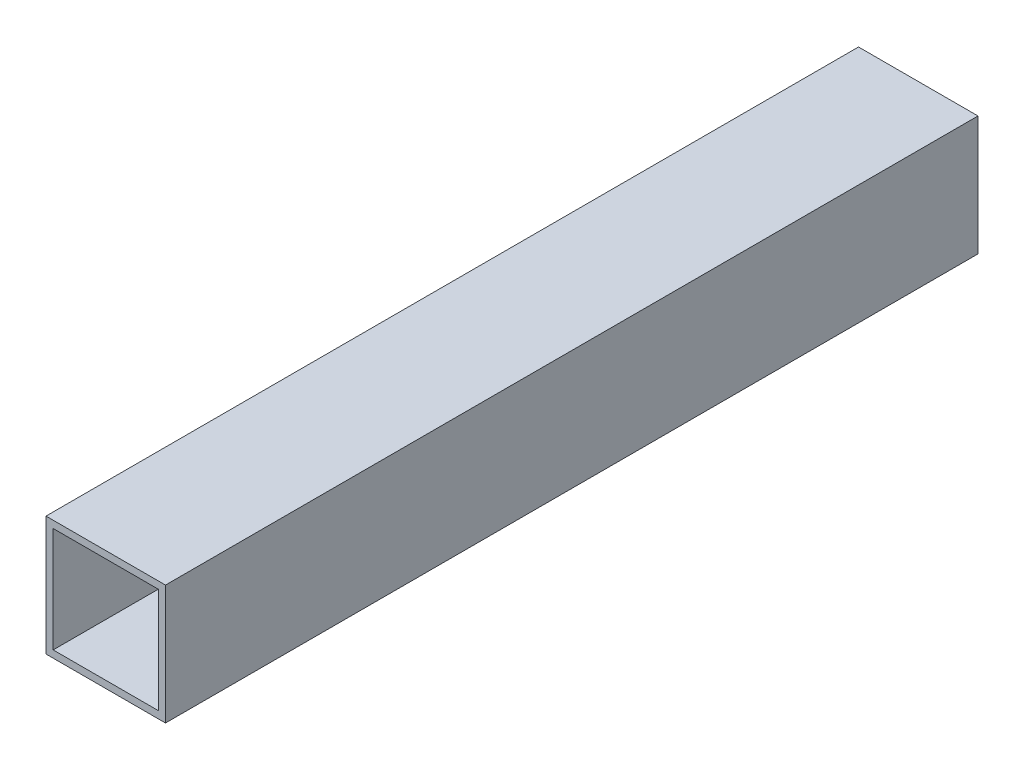
SolidWorks part; units mm, degrees
ref_plane "前视基准面" through (0, 0, 0) normal (0, 0, 1) x (1, 0, 0)
ref_plane "上视基准面" through (0, 0, 0) normal (0, 1, 0) x (1, 0, 0)
ref_plane "右视基准面" through (0, 0, 0) normal (1, 0, 0) x (0, 0, -1)
sketch "草图1" plane through (0, 0, 0) normal (0, 0, 1) x (1, 0, 0)
  line L0 (0, 0) -> (0, 50)
  line L1 (0, 50) -> (50, 50)
  line L2 (50, 50) -> (50, 0)
  line L3 (50, 0) -> (0, 0)
  line L4 (3, 3) -> (3, 47)
  line L5 (3, 47) -> (47, 47)
  line L6 (47, 47) -> (47, 3)
  line L7 (47, 3) -> (3, 3)
  dimension "D1" = 3
extrude "凸台-拉伸2" add sketch "草图1" along normal blind 340
